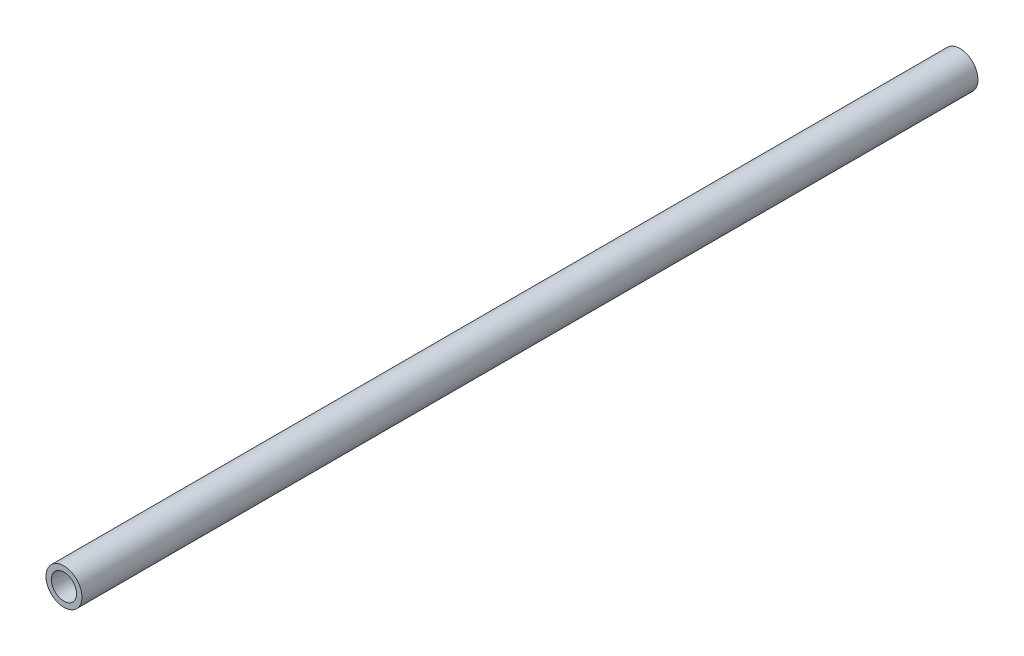
SolidWorks part; units mm, degrees
material "45"
ref_plane "dd" through (0, 0, 0) normal (0, 0, 1) x (1, 0, 0)
ref_plane "Top Plane" through (0, 0, 0) normal (0, 1, 0) x (1, 0, 0)
ref_plane "Right Plane" through (0, 0, 0) normal (1, 0, 0) x (0, 0, -1)
sketch "Sketch4" plane through (0, 0, 0) normal (0, 0, 1) x (1, 0, 0)
  circle A0 centre (16.5, -10.0041) radius 10
  dimension "D1" = 20
extrude "Boss-Extrude1" add sketch "Sketch4" along normal blind 462 and the other way blind 36
sketch "Sketch5" plane through (0, 0, -36) normal (0, 0, -1) x (-1, 0, 0)
  circle A0 centre (-16.5, -10.0041) radius 7
  dimension "D1" = 14
extrude "Cut-Extrude1" cut sketch "Sketch5" against normal through all
